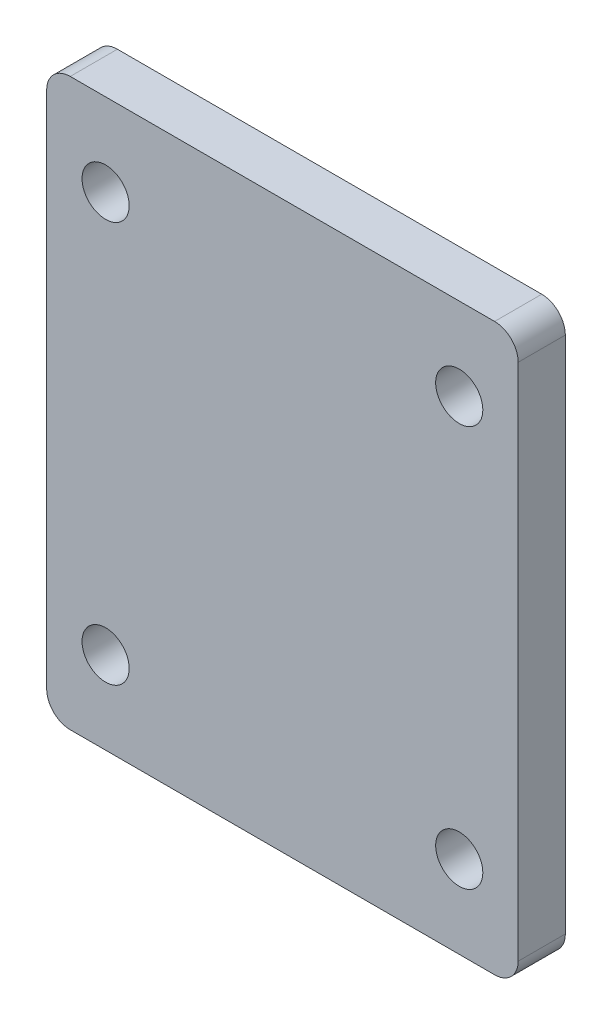
from build123d import *

# Parameters (mm, degrees)
SKETCH1_R           = 5
BOSS_EXTRUDE1_DEPTH = 10


with BuildPart() as part:
    # Sketch1 → Boss-Extrude1 (new body)
    with BuildSketch(Plane.XY):
        with BuildLine():
            Line((5, 0), (95, 0))
            ThreePointArc((95, 0), (98.535533906, -1.464466094), (100, -5))
            Line((100, -5), (100, -115))
            ThreePointArc((100, -115), (98.535533906, -118.535533906), (95, -120))
            Line((95, -120), (5, -120))
            ThreePointArc((5, -120), (1.464466094, -118.535533906), (0, -115))
            Line((0, -115), (0, -5))
            ThreePointArc((0, -5), (1.464466094, -1.464466094), (5, 0))
        make_face()
        with Locations((12.5, -17.5)):
            Circle(SKETCH1_R, mode=Mode.SUBTRACT)
        with Locations((87.5, -17.5)):
            Circle(SKETCH1_R, mode=Mode.SUBTRACT)
        with Locations((87.5, -102.5)):
            Circle(SKETCH1_R, mode=Mode.SUBTRACT)
        with Locations((12.5, -102.5)):
            Circle(SKETCH1_R, mode=Mode.SUBTRACT)
    extrude(amount=BOSS_EXTRUDE1_DEPTH)


solid = part.part
